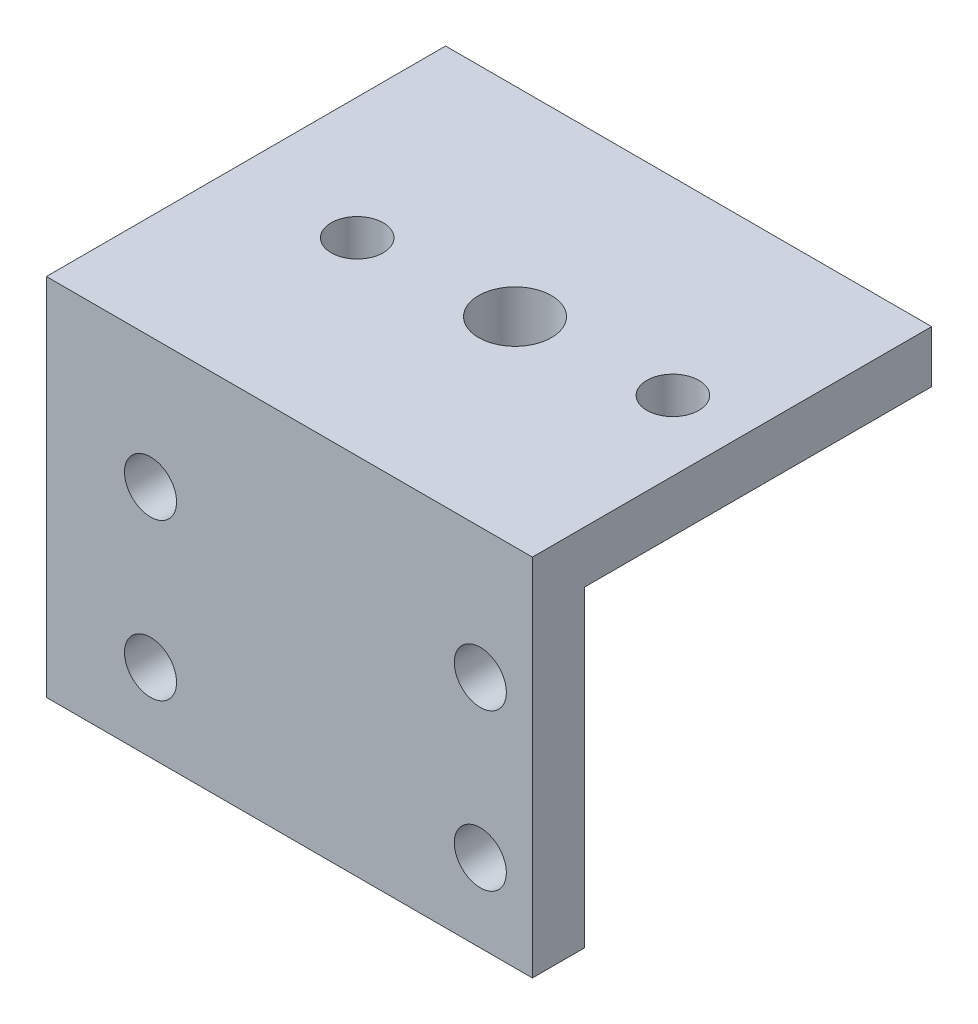
SolidWorks part; units mm, degrees
ref_plane "Front Plane" through (0, 0, 0) normal (0, 0, 1) x (1, 0, 0)
ref_plane "Top Plane" through (0, 0, 0) normal (0, 1, 0) x (1, 0, 0)
ref_plane "Right Plane" through (0, 0, 0) normal (1, 0, 0) x (0, 0, -1)
sketch "Sketch1" plane through (0, 0, 0) normal (0, 0, 1) x (1, 0, 0)
  line L1 (-12.5, -9) -> (12.5, -9)
  line L2 (-12.5, -9) -> (-12.5, 9)
  line L3 (-12.5, 9) -> (12.5, 9)
  line L4 (12.5, -9) -> (12.5, 9)
  line L5 (-12.5, -9) -> (12.5, 9) construction
  line L6 (-12.5, 9) -> (12.5, -9) construction
  circle A0 centre (-9.5, 4.5) radius 1.5
  circle A1 centre (9.5, 4.5) radius 1.5
  circle A2 centre (9.5, -4.5) radius 1.5
  circle A3 centre (-9.5, -4.5) radius 1.5
  point P0 (0, 0)
  dimension "D2" = 3
  dimension "D3" = 3
  dimension "D8" = 3
  dimension "D9" = 3
  dimension "D10" = 19
  dimension "D13" = 3
  dimension "D1" = 18
  dimension "D4" = 4.5
  dimension "D5" = 4.5
  dimension "D6" = 4.5
  dimension "D7" = 9
  dimension "D11" = 25
  dimension "D12" = 3
  dimension "D14" = 19
extrude "Boss-Extrude1" add sketch "Sketch1" along normal blind 3
sketch "Sketch2" plane through (0, 9, 0) normal (0, 1, 0) x (1, 0, 0)
  line L0 (12.5, 0) -> (-12.5, 0) construction
  line L1 (-12.5, -3) -> (12.5, -3)
  line L2 (-12.5, -3) -> (-12.5, 20)
  line L3 (-12.5, 20) -> (12.5, 20)
  line L4 (12.5, -3) -> (12.5, 20)
  circle A0 centre (0, 8.5) radius 2.1
  circle A1 centre (-8.4777, 7.8844) radius 1.5
  circle A2 centre (8.4777, 9.1156) radius 1.5
  dimension "D2" = 4.2
  dimension "D3" = 3
  dimension "D4" = 3
  dimension "D1" = 20
extrude "Boss-Extrude2" add sketch "Sketch2" along normal blind 3
sketch "Sketch3" plane through (-12.5, 0, 0) normal (-1, 0, 0) x (0, 0, 1)
  line L1 (3, 12) -> (-20, 12)
  line L2 (3, 12) -> (3, -9)
  line L3 (3, -9) -> (-20, -9)
  line L4 (-20, 12) -> (-20, -9)
  dimension "D1" = 21
  dimension "D2" = 23
extrude "Boss-Extrude3" add sketch "Sketch3" along normal blind 3
